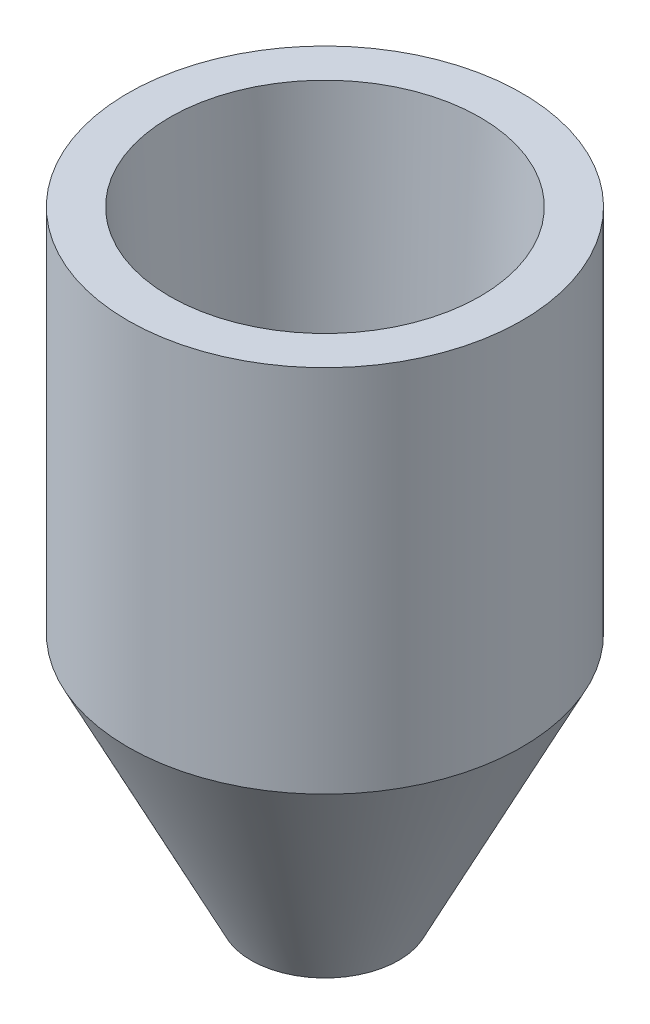
from build123d import *

# Parameters (mm, degrees)
SKETCH_1_R      = 8
EXTRUDE_1_DEPTH = 25
CHAMFER_2_SIZE  = 5
CHAMFER_2_SIZE2 = 10


with BuildPart() as part:
    # 草图1 → 凸台-拉伸1 (new body)
    with BuildSketch(Plane(origin=(0, 0, 0), x_dir=(1, 0, 0), z_dir=(0, 1, 0))):
        with Locations(Location((0, 0, 0), (0, 0, 270))):
            Circle(SKETCH_1_R)
    extrude(amount=EXTRUDE_1_DEPTH)

    # 倒角2
    chamfer_2_edges = [part.edges().sort_by_distance(p)[0] for p in [
        (0, 0, -8),
    ]]
    chamfer_2_side = [part.faces().sort_by_distance(p)[0] for p in [
        (0, 0, 0),
    ]]
    chamfer(chamfer_2_edges, length=CHAMFER_2_SIZE, length2=CHAMFER_2_SIZE2, reference=chamfer_2_side[0])

    # 草图3 → 切除-旋转1 (revolve, cut)
    with BuildSketch(Plane(origin=(0, 0, 0), x_dir=(0, 0, -1), z_dir=(1, 0, 0)), mode=Mode.PRIVATE) as cut_revolve_1_sk:
        Polygon((6.3, 25), (5.75, 14), (0, 14), (0, 25), align=None)
    revolve(cut_revolve_1_sk.sketch.rotate(Axis((0, 25, 0), (0, -1, 0)), 180), axis=Axis((0, 25, 0), (0, -1, 0)), mode=Mode.SUBTRACT)


solid = part.part
